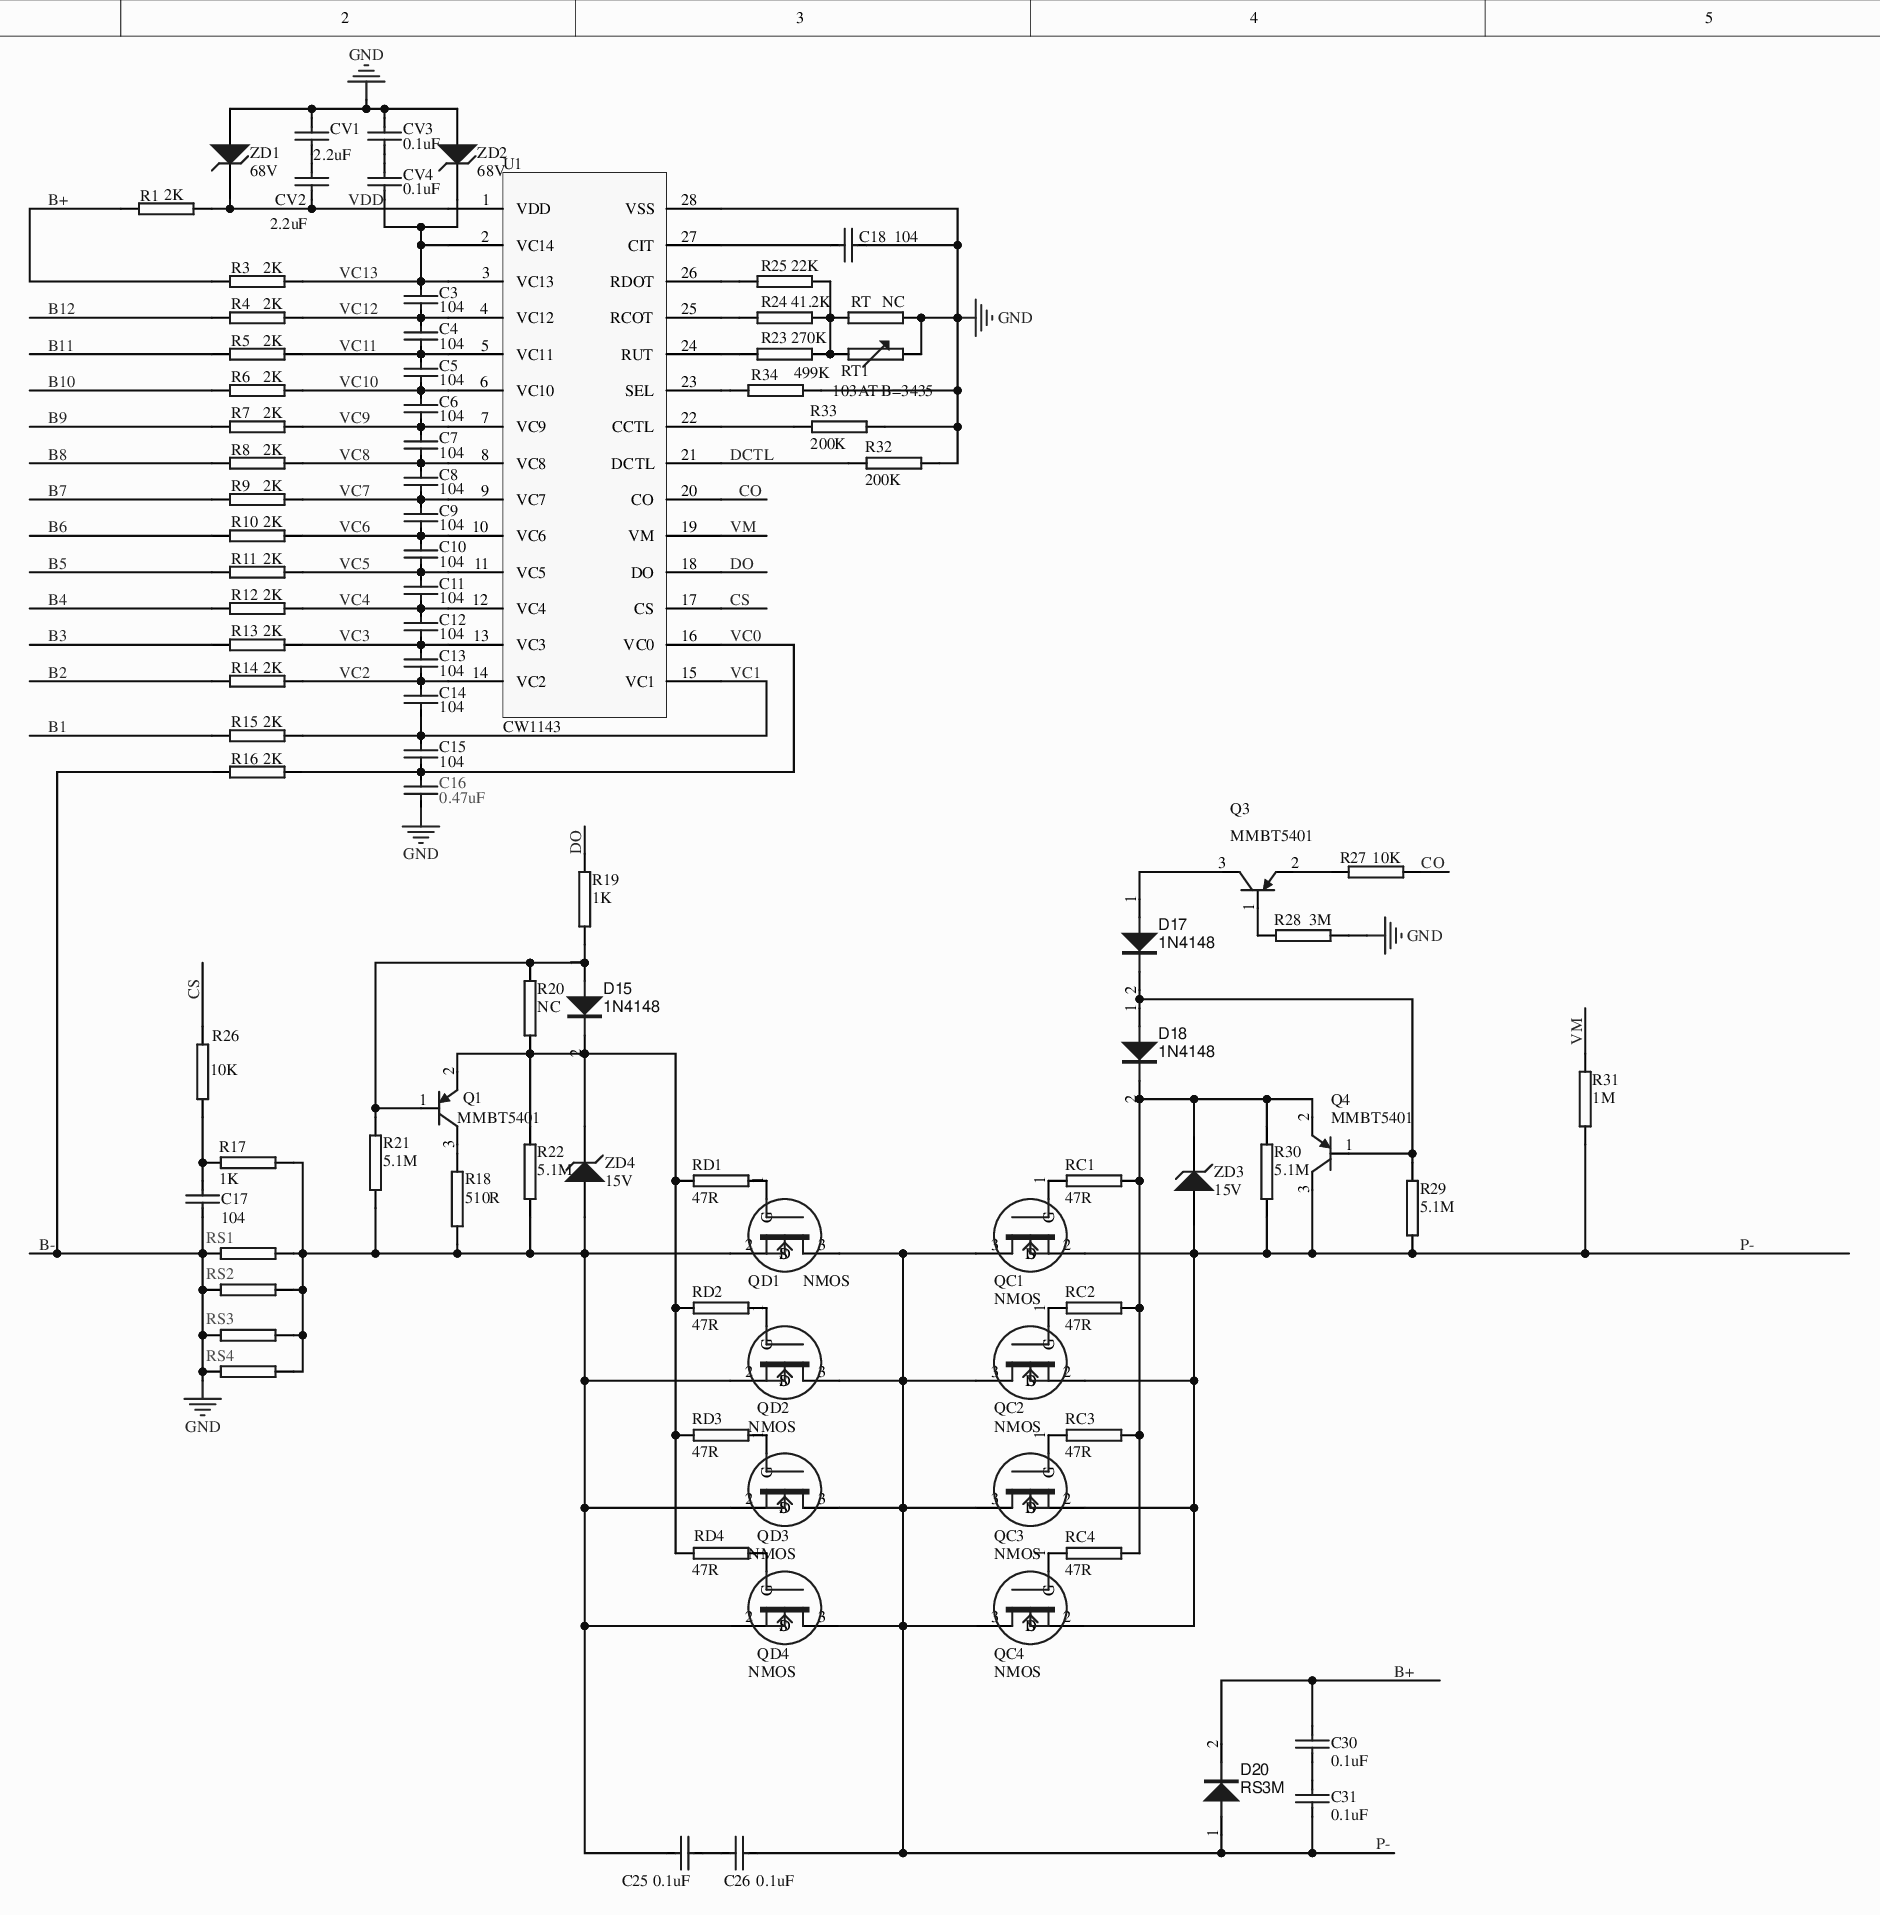
[diagram p0: MISC84297-5.SchDoc]
# Altium project MISC84297-3.PrjPcb
1 sheet, 91 parts. Net scope: global (net labels, ports and power ports of the same name join across sheets).
Board file: MISC84297.PcbDoc

## Sheet MISC84297-5.SchDoc
size 508 x 281 mm; SheetNumber: 1; SheetTotal: 1; PageSetup: Record=PageOptions¦CenterHorizontal=True¦CenterVertical=True¦PrintScale=0.77¦XCorrection=1.00¦YCorrection=1.00¦PrintKind=0¦BorderSize=5000000¦LeftOffset=0¦BottomOffset=0¦Orientation=2¦PaperLength=1000¦PaperWidth=1000¦Scale=100¦PaperSource=7¦PrintQuality=-3¦MediaType=1¦DitherType=10¦PrintScaleMode=1¦PaperKind=A4¦PaperIndex=9

### Parts
C3  104  [CAP0603]
C4  104  [CAP0603]
C5  104  [CAP0603]
C6  104  [CAP0603]
C7  104  [CAP0603]
C8  104  [CAP0603]
C9  104  [CAP0603]
C10  104  [CAP0603]
C11  104  [CAP0603]
C12  104  [CAP0603]
C13  104  [CAP0603]
C14  104  [CAP0603]
C15  104  [CAP0603]
C16  0.47uF  [CAP0603]
C17  104  [CAP0603]
C18  104  [CAP0603]
C25  0.1uF  [CAP0603]
C26  0.1uF  [CAP0603]
C30  0.1uF  [CAP0603]
C31  0.1uF  [CAP0603]
CV1  2.2uF  [CAP0805]
CV2  2.2uF  [CAP0805]
CV3  0.1uF  [CAP0603]
CV4  0.1uF  [CAP0603]
D15  1N4148  [SOD323]
D17  1N4148  [SOD323]
D18  1N4148  [SOD323]
D20  RS3M  [SMC]
Q1  MMBT5401  [SOT-23-3]
Q3  MMBT5401  [SOT-23-3]
Q4  MMBT5401  [SOT-23-3]
QC1  NMOS  [TOLL_123]
QC2  NMOS  [TOLL_123]
QC3  NMOS  [TOLL_123]
QC4  NMOS  [TOLL_123]
QD1  NMOS  [TOLL_123]
QD2  NMOS  [TOLL_123]
QD3  NMOS  [TOLL_123]
QD4  NMOS  [TOLL_123]
R1  2K  [RES0805]
R3  2K  [RES0603]
R4  2K  [RES0603]
R5  2K  [RES0603]
R6  2K  [RES0603]
R7  2K  [RES0603]
R8  2K  [RES0603]
R9  2K  [RES0603]
R10  2K  [RES0603]
R11  2K  [RES0603]
R12  2K  [RES0603]
R13  2K  [RES0603]
R14  2K  [RES0603]
R15  2K  [RES0603]
R16  2K  [RES0603]
R17  1K  [RES0603]
R18  510R  [RES0603]
R19  1K  [RES0603]
R20  NC  [RES0603]
R21  5.1M  [RES0603]
R22  5.1M  [RES0603]
R23  270K  [RES0603]
R24  41.2K  [RES0603]
R25  22K  [RES0603]
R26  10K  [RES0603]
R27  10K  [RES0603]
R28  3M  [RES0603]
R29  5.1M  [RES0603]
R30  5.1M  [RES0603]
R31  1M  [RES0603]
R32  200K  [RES0603]
R33  200K  [RES0603]
R34  499K  [RES0603]
RC1  47R  [RES0603]
RC2  47R  [RES0603]
RC3  47R  [RES0603]
RC4  47R  [RES0603]
RD1  47R  [RES0603]
RD2  47R  [RES0603]
RD3  47R  [RES0603]
RD4  47R  [RES0603]
RS1  (no value)  [2512]
RS2  (no value)  [2512]
RS3  (no value)  [2512]
RS4  (no value)  [2512]
RT  NC  [RES0603]
RT1  103AT B=3435  [WK]
U1  CW1143  [SSOP-28-0.635]
ZD1  68V  [SOD123]
ZD2  68V  [SOD123]
ZD3  15V  [SOD323]
ZD4  15V  [SOD323]

### Nets
B-: C16.2 C17.2 C18.2 CV1.1 CV3.1 R16.1 R28.1 R32.2 R33.2 R34.2 RS1.2 RS2.2 RS3.2 RS4.2 RT.2 RT1.2 U1.28(VSS) ZD1.1(A) ZD2.1(A)  [also labelled GND]
B1: R15.1
B2: R14.1
B3: R13.1
B4: R12.1
B5: R11.1
B6: R10.1
B7: R9.1
B8: R8.1
B9: R7.1
B10: R6.1
B11: R5.1
B12: R4.1
B+: C30.2 D20.2(K) R1.1 R3.1
CO: R27.2 U1.20(CO)
CS: R26.2 U1.17(CS)
DCTL: R32.1 U1.21(DCTL)
DO: R19.1 U1.18(DO)
P-: C26.2 C31.1 D20.1(A) Q4.3(C) QC1.2(S) QC1.3(D) QC2.2(S) QC2.3(D) QC3.2(S) QC3.3(D) QC4.2(S) QC4.3(D) QD1.3(D) QD2.3(D) QD3.3(D) QD4.3(D) R29.2 R30.2 R31.2 ZD3.1(A)
VC0: C15.2 C16.1 R16.2 U1.16(VC0)
VC1: C14.2 C15.1 R15.2 U1.15(VC1)
VC2: C13.2 C14.1 R14.2 U1.14(VC2)
VC3: C12.2 C13.1 R13.2 U1.13(VC3)
VC4: C11.2 C12.1 R12.2 U1.12(VC4)
VC5: C10.2 C11.1 R11.2 U1.11(VC5)
VC6: C9.2 C10.1 R10.2 U1.10(VC6)
VC7: C8.2 C9.1 R9.2 U1.9(VC7)
VC8: C7.2 C8.1 R8.2 U1.8(VC8)
VC9: C6.2 C7.1 R7.2 U1.7(VC9)
VC10: C5.2 C6.1 R6.2 U1.6(VC10)
VC11: C4.2 C5.1 R5.2 U1.5(VC11)
VC12: C3.2 C4.1 R4.2 U1.4(VC12)
VC13: C3.1 CV4.2 R3.2 U1.2(VC14) U1.3(VC13) ZD2.2(K)
VDD: CV2.2 R1.2 U1.1(VDD) ZD1.2(K)
VM: R31.1 U1.19(VM)
NetC17_1: C17.1 R17.1 R26.1
NetC18_1: C18.1 U1.27(CIT)
NetC25_1: C25.1 QD1.2(S) QD2.2(S) QD3.2(S) QD4.2(S) R17.2 R18.2 R21.2 R22.2 RS1.1 RS2.1 RS3.1 RS4.1 ZD4.1(A)
NetC25_2: C25.2 C26.1
NetC30_1: C30.1 C31.2
NetCV1_2: CV1.2 CV2.1
NetCV3_2: CV3.2 CV4.1
NetD15_1: D15.1(A) Q1.1(B) R19.2 R20.1 R21.1
NetD15_2: D15.2(K) Q1.2(E) R20.2 R22.1 RD1.1 RD2.1 RD3.1 RD4.1 ZD4.2(K)
NetD17_1: D17.1(A) Q3.3(C)
NetD17_2: D17.2(K) D18.1(A) Q4.1(B) R29.1
NetD18_2: D18.2(K) Q4.2(E) R30.1 RC1.1 RC2.1 RC3.1 RC4.1 ZD3.2(K)
NetQ1_3: Q1.3(C) R18.1
NetQ3_1: Q3.1(B) R28.2
NetQ3_2: Q3.2(E) R27.1
NetQC1_1: QC1.1(G) RC1.2
NetQC2_1: QC2.1(G) RC2.2
NetQC3_1: QC3.1(G) RC3.2
NetQC4_1: QC4.1(G) RC4.2
NetQD1_1: QD1.1(G) RD1.2
NetQD2_1: QD2.1(G) RD2.2
NetQD3_1: QD3.1(G) RD3.2
NetQD4_1: QD4.1(G) RD4.2
NetR23_1: R23.1 U1.24(RUT)
NetR23_2: R23.2 R24.2 R25.2 RT.1 RT1.1
NetR24_1: R24.1 U1.25(RCOT)
NetR25_1: R25.1 U1.26(RDOT)
NetR33_1: R33.1 U1.22(CCTL)
NetR34_1: R34.1 U1.23(SEL)

### Library data of the parts
C3-C18 C25 C26 C30 C31 CV1-CV4 = CAP
D15 D17 D18 D20 = DIODE
Q1 Q3 Q4 = PNP: PNP Bipolar Transistor; Published: 8-Jun-2000; LatestRevisionDate: 29-May-2009; LatestRevisionNote: IPC-7351 Footprint Added.; PackageVersion: Aug-1999; PackageReference: SOT-23B; PackageDescription: 3-Pin SOT-23 Package 0.95 mm Pitch, 2.4 mm Lead Span; Publisher: Altium Limited
R1 R3-R34 RC1-RC4 RD1-RD4 RS1-RS4 RT = RES
RT1 = RT1
ZD1-ZD4 = D Zener: Zener Diode; Published: 8-Jun-2000; LatestRevisionDate: 17-Jul-2002; LatestRevisionNote: Re-released for DXP Platform.; PackageReference: DIODE-0.7; PackageDescription: Diode, Thru-Hole; 2 Leads; 0.7 in Pin Spacing; Publisher: Altium Limited